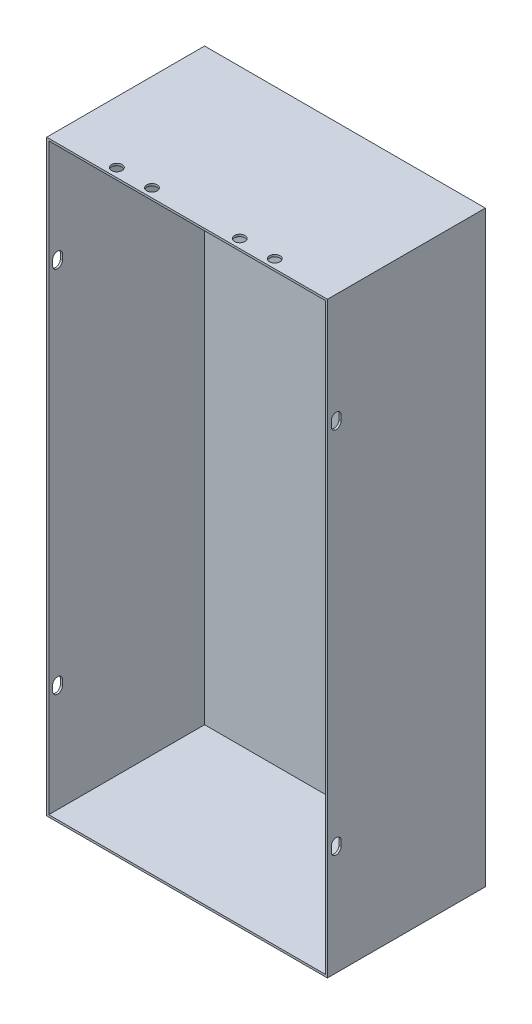
SolidWorks part; units mm, degrees
ref_plane "Front Plane" through (0, 0, 0) normal (0, 0, 1) x (1, 0, 0)
ref_plane "Top Plane" through (0, 0, 0) normal (0, 1, 0) x (1, 0, 0)
ref_plane "Right Plane" through (0, 0, 0) normal (1, 0, 0) x (0, 0, -1)
sketch "Sketch1" plane through (0, 0, 0) normal (0, 0, 1) x (1, 0, 0)
  line L1 (-80, -167.5) -> (80, -167.5)
  line L2 (-80, -167.5) -> (-80, 167.5)
  line L3 (-80, 167.5) -> (80, 167.5)
  line L4 (80, -167.5) -> (80, 167.5)
  line L5 (-80, -167.5) -> (80, 167.5) construction
  line L6 (-80, 167.5) -> (80, -167.5) construction
  point P0 (0, 0)
  dimension "D1" = 160
  dimension "D2" = 335
extrude "Boss-Extrude1" add sketch "Sketch1" along normal blind 90
shell "Shell1" thickness 1.2
sketch "Sketch2" plane through (0, 167.5, 0) normal (0, 1, 0) x (1, 0, 0)
  line L0 (0, 0) -> (0, -110.317) construction
  line L1 (80, 0) -> (-80, 0) construction
  line L2 (80, -90) -> (-80, -90) construction
  circle A0 centre (-45, -85) radius 3
  circle A1 centre (-25, -85) radius 3
  circle A2 centre (25, -85) radius 3
  circle A3 centre (45, -85) radius 3
  dimension "D1" = 50
  dimension "D5" = 6
  dimension "D3" = 5
  dimension "D4" = 5
  dimension "D2" = 90
extrude "Cut-Extrude1" cut sketch "Sketch2" against normal blind 10
sketch "Sketch3" plane through (-80, 0, 0) normal (-1, 0, 0) x (0, 0, 1)
  line L0 (85, 106.5) -> (85, 103.5) construction
  line L1 (87.8, 106.5) -> (87.8, 103.5)
  line L2 (82.2, 106.5) -> (82.2, 103.5)
  line L4 (0, 0) -> (120.859, 0) construction
  line L5 (85, -106.5) -> (85, -103.5) construction
  line L6 (87.8, -106.5) -> (87.8, -103.5)
  line L7 (82.2, -106.5) -> (82.2, -103.5)
  line L8 (90, 167.5) -> (90, -167.5) construction
  arc A0 (87.8, 106.5) -> (82.2, 106.5) centre (85, 106.5) ccw
  arc A1 (82.2, 103.5) -> (87.8, 103.5) centre (85, 103.5) ccw
  arc A2 (87.8, -106.5) -> (82.2, -106.5) centre (85, -106.5) cw
  arc A3 (82.2, -103.5) -> (87.8, -103.5) centre (85, -103.5) cw
  point P2 (85, 105)
  point P7 (85, 109.3)
  point P8 (85, 100.7)
  point P16 (85, -105)
  dimension "D2" = 8.6
  dimension "D4" = 210
  dimension "D1" = 5.6
  dimension "D3" = 5
extrude "Cut-Extrude2" cut sketch "Sketch3" against normal through all
